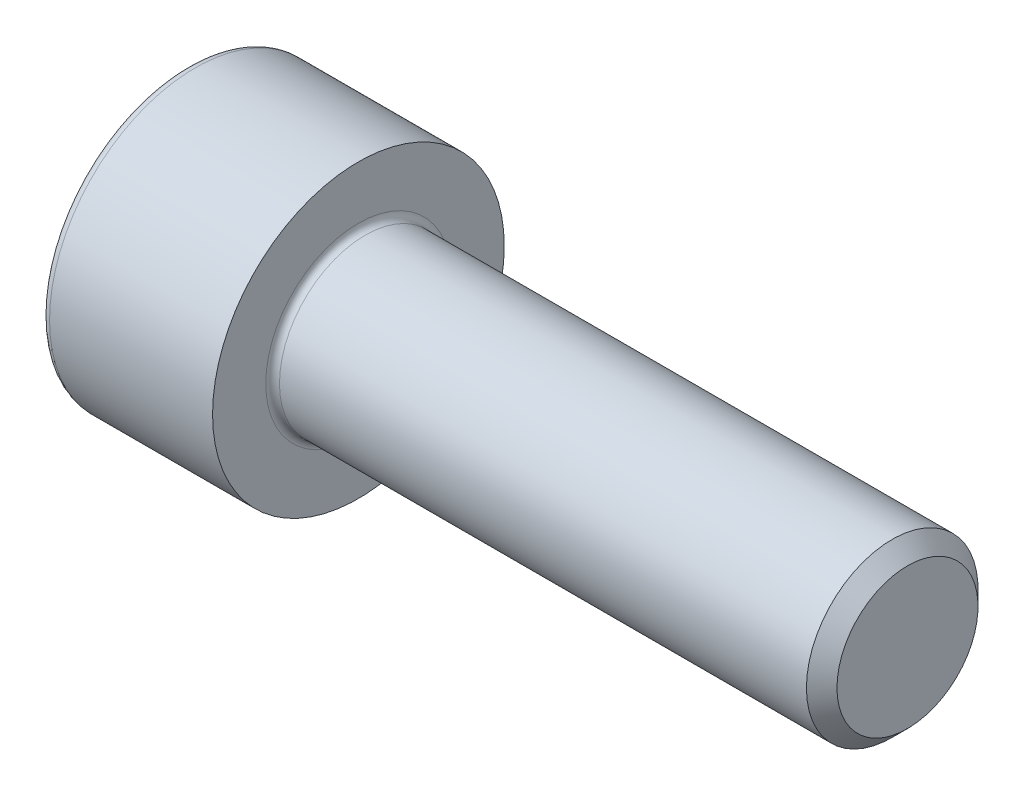
SolidWorks part; units mm, degrees
revolve "Base-Revolve" add sketch "BodySke"
sketch "BodySke" plane through (0, 0, 0) normal (0, 0, 1) x (1, 0, 0)
  line L0 (0, 0) -> (0, 4.25)
  line L1 (0, 4.25) -> (5, 4.25)
  line L2 (5, 4.25) -> (5, 2.5)
  line L3 (5, 2.5) -> (20.555, 2.5)
  line L4 (21, 2.055) -> (21, 0)
  line L5 (21, 0) -> (0, 0)
  line L6 (-31.75, 0) -> (127, 0) construction
  line L8 (21, 2.055) -> (20.555, 2.5)
  line L10 (21, -2.055) -> (20.555, -2.5) construction
  line L11 (5.8, 9.525) -> (5.8, 3.175) construction
  line L12 (5, 9.525) -> (5, 3.175) construction
  line L13 (-39, 9.525) -> (-39, 3.175) construction
cosmetic thread "ThreadCosmetic" [suppressed]
fillet "Fillet1" radius 0.2 1 edges at (5, 0, 2.5)
fillet "Fillet2" radius 0.25 1 edges at (0, 0, 4.25)
ref_plane "Plane1" through (0, 0, 0) normal (0, 0, 1) x (1, 0, 0)
ref_plane "Plane2" through (0, 0, 0) normal (0, 1, 0) x (1, 0, 0)
ref_plane "Plane3" through (0, 0, 0) normal (1, 0, 0) x (0, 0, -1)
sketch "Sketch2" plane through (0, 0, 0) normal (0, 0, 1) x (1, 0, 0)
  line L0 (0, 2.042) -> (2.5, 2.042)
  line L1 (2.5, 2.042) -> (3.6789, 0)
  line L2 (-31.75, 0) -> (127, 0) construction
  line L3 (3.6789, 0) -> (0, 0)
  line L4 (0, 0) -> (0, 2.042)
  line L6 (0, 0) -> (47.625, 0) construction
revolve "Hex-PreBroach" cut sketch "Sketch2" angle 360 about L6
sketch "Sketch3" plane through (0, 0, 0) normal (-1, 0, 0) x (0, 0.5, 0.866)
  line L0 (1.1789, 2.042) -> (-1.1789, 2.042)
  line L1 (-1.1789, 2.042) -> (-2.3579, 0)
  line L2 (1.1789, 2.042) -> (2.3579, 0)
  line L3 (1.1789, -2.042) -> (2.3579, 0)
  line L4 (1.1789, -2.042) -> (-1.1789, -2.042)
  line L5 (-1.1789, -2.042) -> (-2.3579, 0)
extrude "Hex" cut sketch "Sketch3" against normal blind 2.5
sketch "ThdSchSke" plane through (0, 0, 0) normal (0, 0, 1) x (1, 0, 0)
  line L0 (7.4, -2.055) -> (7.0884, -2.5)
  line L1 (7.4, -2.055) -> (7.7116, -2.5)
  line L2 (7.7116, -2.5) -> (7.7116, -3.125)
  line L3 (-3.175, 0) -> (5.1513, 0) construction
  line L4 (0, 4) -> (0, -4) construction
  line L5 (7.7116, -3.125) -> (7.0884, -3.125)
  line L6 (7.0884, -3.125) -> (7.0884, -2.5)
revolve "ThreadSchematic" [suppressed] cut sketch "ThdSchSke" angle 360 about L3
pattern_linear "ThdSchPat" [suppressed]
equation "\"D2@Sketch3\" = \"Hex_size@Sketch3\" / 2"
equation "\"D1@Sketch3\" = \"Hex_size@Sketch3\" / 2"
equation "\"D1@Sketch2\" = \"Hex_size@Sketch3\" / 2"
equation "\"Thread_minor@ThreadCosmetic\"  =  \"Minor_dia@BodySke\""
equation "\"Depth@Sketch2\" =  \"Key_eng@Hex\""
equation "\"Thread_length@ThreadCosmetic\" = ((sgn( (\"Length@BodySke\" - \"Advance@BodySke\" * 3.0) - \"Thread_nom@BodySke\" )-1)*( (\"Length@BodySke\" - \"Advance@BodySke\" * 3.0) - \"Thread_nom@BodySke\" ))/-2+ \"Thread_nom@BodySke\""
equation "\"Thread_minor@ThdSchSke\" = \"Minor_dia@BodySke\""
equation "\"Diameter@ThdSchSke\" = \"Diameter@BodySke\""
equation "\"Overcut@ThdSchSke\" = \"Diameter@BodySke\" * 1.25"
equation "\"Start@ThdSchSke\" = \"Head_ht@BodySke\" + \"Length@BodySke\" - \"Thread_length@ThreadCosmetic\"  '---Non-countersunk---"
equation "\"Num_threads@ThdSchPat\" = int( \"Thread_length@ThreadCosmetic\" / \"Advance@BodySke\" + 0.999 )  + 1"
equation "\"Advance@ThdSchPat\" = \"Thread_length@ThreadCosmetic\" /  (\"Num_threads@ThdSchPat\" - 1) 'relax it"
equation "\"Num_threads@ThdSchPat\" = \"Num_threads@ThdSchPat\" - sgn( \"Num_threads@ThdSchPat\" - 1) '---chamfered tips only---"
